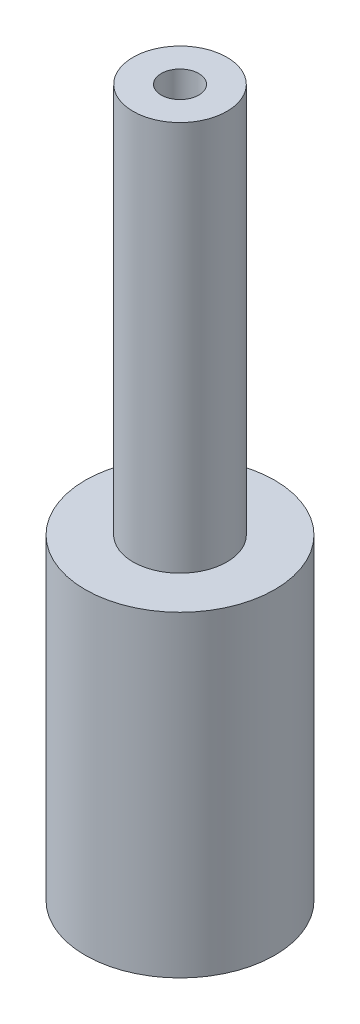
from build123d import *


with BuildPart() as part:
    # Sketch1 → Revolve2 (revolve)
    with BuildSketch(Plane.XY, mode=Mode.PRIVATE) as revolve2_sk:
        Polygon((-1.25, 8.44), (-1.25, 18.84), (-0.5, 18.84), (-0.5, 0), (-2.525, 0), (-2.525, 8.44), align=None)
    revolve(revolve2_sk.sketch.rotate(Axis((0, 23.646410138, 0), (0, -1, 0)), 270), axis=Axis((0, 23.646410138, 0), (0, -1, 0)))


solid = part.part
